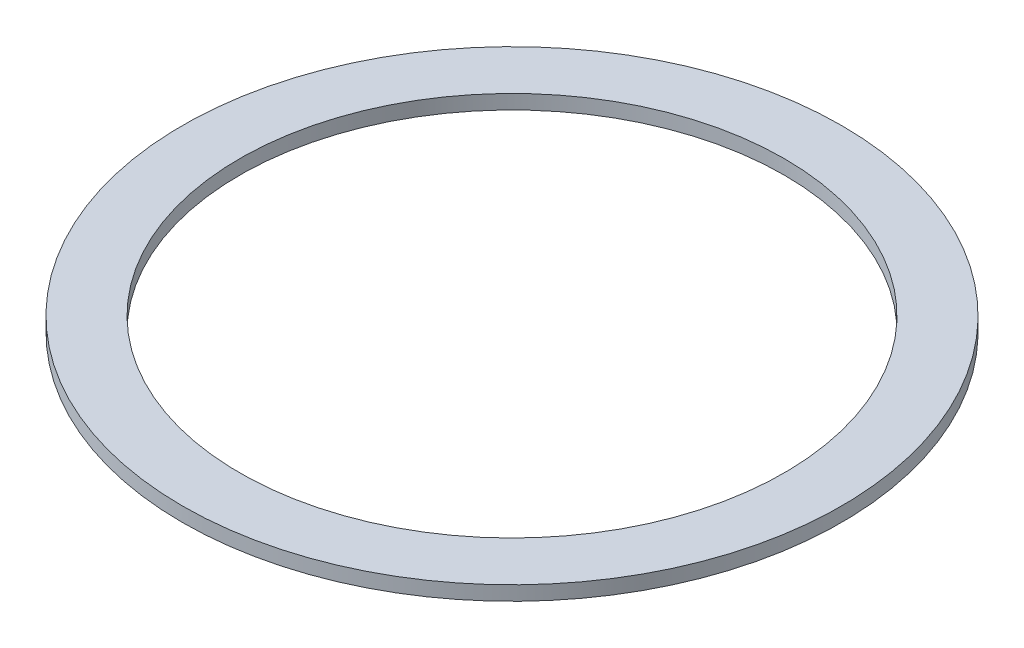
from build123d import *

# Parameters (mm, degrees)
SKETCH1_W = 4
SKETCH1_H = 1


with BuildPart() as part:
    # Sketch1 → Revolve1 (revolve)
    with BuildSketch(Plane.XY, mode=Mode.PRIVATE) as revolve1_sk:
        with Locations((21, 0.5)):
            Rectangle(SKETCH1_W, SKETCH1_H)
    revolve(revolve1_sk.sketch.rotate(Axis((0, 0, 0), (0, 1, 0)), 90), axis=Axis((0, 0, 0), (0, 1, 0)))


solid = part.part
